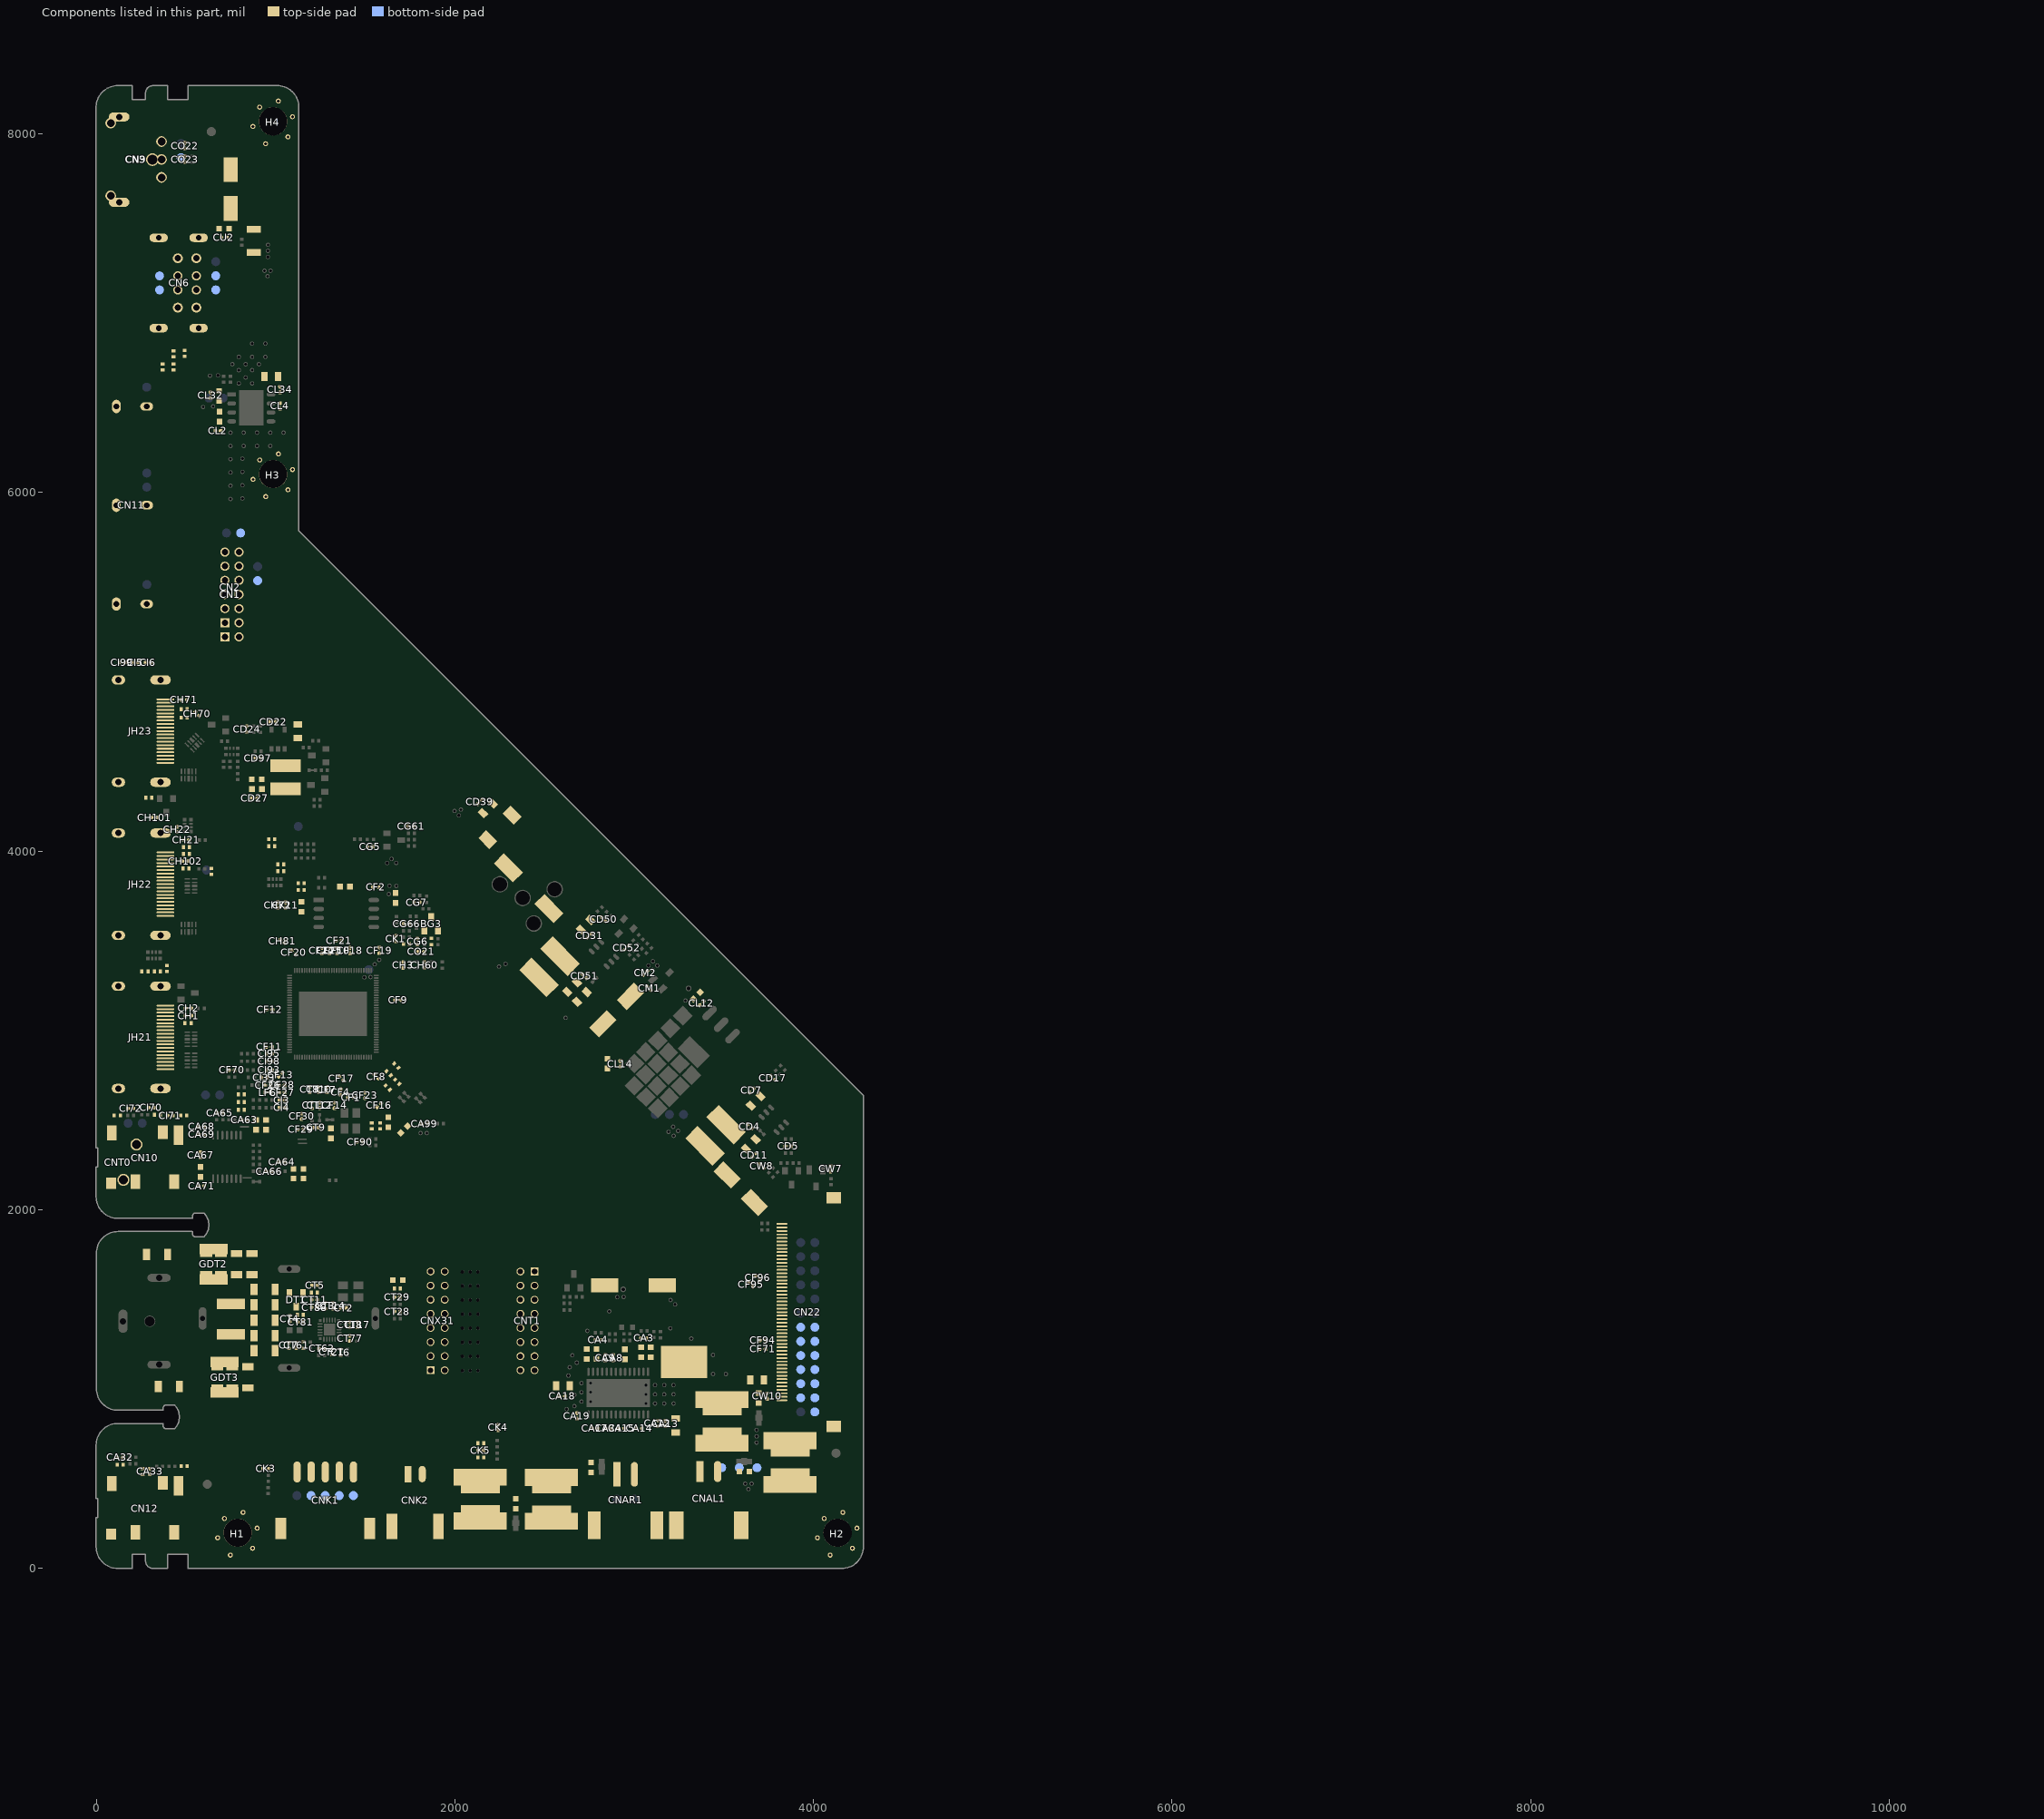
[diagram p0: the components of this part, seen from the top]
# Altium PCB MISC105950.PcbDoc (part 2 of 15)
Units mil, origin at the board's own origin, x right, y up, seen from the top; angles counter-clockwise.
Board outline 4280.62 x 8272.76 mil, 2 copper layers (TopLayer, BottomLayer), stack 61.855 mil thick; 541 components, 268 nets, 2324 pads, 1157 vias.

## Components (designator, comment, footprint, x,y, rotation, side; value= is the part's Value field where it differs from the comment) (continued)
BG3 "NC/General-purpose transistor, Dynatron, NPN, 0.2A, 40V, 30-300, SOT-23, MMBT3904(f≥350MHz), BLUE ROCKET" SOT-23 1866.5,3595 r180 top
BLON "TEST" TP 803.5,5774.51 r90 bottom
CA1 "Ceramic capacitor, CAP MC, 25V, 10uF, ±10%, X5R, 0805, SMD, TP" C0805 3231,795 r270 top
CA2 "NC/Ceramic capacitor, CAP MC, 25V, 10uF, ±10%, X5R, 0805, SMD, TP" C0805 2601.5,1017 r180 top
CA3 "3300pF-0402-X7R-±10%-50V" C0402 3053,1282.5 r0 top
CA4 "3300pF-0402-X7R-±10%-50V" C0402 2799.02,1273.23 r0 top
CA5 "Ceramic capacitor, CAP MC, 25V, 0.22uF, ±10%, X7R, 0603, SMD, TP" C0603 3092,1204 r270 top
CA6 "Ceramic capacitor, CAP MC, 25V, 0.22uF, ±10%, X7R, 0603, SMD, TP" C0603 3038,1204 r270 top
CA7 "Ceramic capacitor, CAP MC, 25V, 1uF, ±10%, X5R, 0603, SMD, TP" C0603 2947,1192.5 r90 top
CA8 "1uF-0402-X5R-±20%-16V" C0402 2881.84,1172.5 r270 top
CA9 "NC/1uF-0402-X5R-±20%-16V" C0402 2837.44,1172.5 r270 top
CA10 "Ceramic capacitor, CAP MC, 25V, 0.22uF, ±10%, X7R, 0603, SMD, TP" C0603 2788.94,1193.5 r270 top
CA11 "Ceramic capacitor, CAP MC, 25V, 0.22uF, ±10%, X7R, 0603, SMD, TP" C0603 2734.94,1193.5 r270 top
CA12 "NC/Ceramic capacitor, CAP MC, 25V, 0.1uF, ±20%, X5R, 0402, SMD, TP" C0402 3130.5,806.5 r270 top
CA13 "1000pF-0402-X7R-±10%-50V" C0402 3173,806.16 r270 top
CA14 "0.22uF-0402-X5R-±10%-16V" C0402 3027,779 r180 top
CA15 "0.22uF-0402-X5R-±10%-16V" C0402 2929,779 r0 top
CA17 "0.22uF-0402-X5R-±10%-16V" C0402 2781,779 r0 top
CA18 "NC/Ceramic capacitor, CAP MC, 25V, 0.1uF, ±20%, X5R, 0402, SMD, TP" C0402 2598.5,958.5 r180 top
CA19 "1000pF-0402-X7R-±10%-50V" C0402 2680,848.5 r270 top
CA20 "Ceramic capacitor, CAP MC, 25V, 1uF, ±10%, X5R, 0603, SMD, TP" C0603 3693.5,947.5 r270 top
CA21 "Ceramic capacitor, CAP MC, 25V, 1uF, ±10%, X5R, 0603, SMD, TP" C0603 3613.5,537.5 r180 top
CA22 "Ceramic capacitor, CAP MC, 25V, 1uF, ±10%, X5R, 0603, SMD, TP" C0603 2759,561 r270 top
CA23 "Ceramic capacitor, CAP MC, 25V, 1uF, ±10%, X5R, 0603, SMD, TP" C0603 2339.05,359 r90 top
CA29 "Ceramic capacitor, CAP MC, 6.3V, 22uF, ±20%, X5R, 0603, SMD, TP" C0603 1125.98,2226.34 r0 top
CA31 "NC/NC/Ceramic capacitor, CAP MC, 6.3V, 10uF, ±20%, X5R, 0603, SMD, TP" C0603 917.13,2445 r0 top
CA32 "NC/6800pF-0402-X7R-±10%-50V" C0402 131.5,617 r180 top
CA33 "NC/6800pF-0402-X7R-±10%-50V" C0402 297,538.5 r90 top
CA34 "0.22uF-0402-X5R-±10%-16V" C0402 2855.5,779 r180 top
CA59 "NC/NC/Ceramic capacitor, CAP MC, 6.3V, 10uF, ±20%, X5R, 0603, SMD, TP" C0603 1125.98,2172.75 r0 top
CA60 "Ceramic capacitor, CAP MC, 6.3V, 22uF, ±20%, X5R, 0603, SMD, TP" C0603 917.13,2499.75 r0 top
CA63 "NC/1uF-0402-X5R-±20%-6.3V" C0402 824.77,2501 r180 top
CA64 "NC/1uF-0402-X5R-±20%-6.3V" C0402 1035,2266 r180 top
CA65 "NC/NC/?" C0402 688,2539.5 r180 top
CA66 "NC/NC/?" C0402 962.74,2213.5 r180 top
CA67 "NC/1uF-0402-X5R-±20%-6.3V" C0402 580,2304 r90 top
CA68 "NC/1uF-0402-X5R-±20%-6.3V" C0402 585.66,2461.69 r180 top
CA69 "NC/0.1uF-0402-X7R-±10%-16V" C0402 585.66,2420 r180 top
CA70 "NC/Ceramic capacitor, CAP MC, 6.3V, 10uF, ±20%, X5R, 0603, SMD, TP" C0603 579.5,2209.88 r90 top
CA71 "NC/0.1uF-0402-X5R-±20%-16V" C0402 585.35,2131.5 r180 top
CA99 "Ceramic capacitor, CAP MC, 6.3V, 1uF, ±20%, X5R, 0402, SMD, TP" C0402 1829.35,2478.5 r180 top
CD4 "NC/0.1uF-0402-X7R-±10%-16V" C0402 3643.54,2463.96 r315 top
CD5 "NC/Ceramic capacitor, CAP MC, 50V, 1000pF, ±10%, X7R, 0402, SMD, TP" C0402 3858.27,2353.5 r180 top
CD7 "NC/NC/Ceramic capacitor, CAP MC, 25V, 0.1uF, ±20%, X5R, 0402, SMD, TP" C0402 3654.54,2664.04 r45 top
CD11 "NC/NC/0.1uF-0402-X5R-±20%-16V" C0402 3669.5,2303.5 r225 top
CD17 "NC/NC/Ceramic capacitor, CAP MC, 25V, 0.1uF, ±20%, X5R, 0402, SMD, TP" C0402 3773.5,2734.5 r315 top
CD22 "NC/0.1uF-0402-X5R-±20%-16V" C0402 984.65,4721.5 r0 top
CD24 "NC/3300pF-0402-X7R-±10%-50V" C0402 838,4680.5 r270 top
CD25 "10uF-0603-X5R-±20%-6.3V" C0603 893.69,4399.5 r0 top
CD26 "10uF-0603-X5R-±20%-6.3V" C0603 894.75,4345.41 r0 top
CD27 "NC/0.1uF-0402-X5R-±20%-16V" C0402 882.15,4295.5 r0 top
CD30 "Ceramic capacitor, CAP MC, 25V, 10uF, ±10%, X5R, 0805, SMD, TP" C0805 2728,3588.5 r225 top
CD31 "NC/Ceramic capacitor, CAP MC, 25V, 0.1uF, ±20%, X5R, 0402, SMD, TP" C0402 2749,3527.5 r45 top
CD39 "NC/Ceramic capacitor, CAP MC, 25V, 0.1uF, ±20%, X5R, 0402, SMD, TP" C0402 2138.5,4274.5 r225 top
CD50 "NC/Ceramic capacitor, CAP MC, 25V, 0.1uF, ±20%, X5R, 0402, SMD, TP" C0402 2829,3619 r315 top
CD51 "0.1uF-0402-X7R-±10%-16V" C0402 2721.5,3302 r315 top
CD52 "Ceramic capacitor, CAP MC, 50V, 1000pF, ±10%, X7R, 0402, SMD, TP" C0402 2956.72,3460.1 r45 top
CD53 "10uF-0805-X5R-±20%-16V" C0805 2653.1,3240.4 r45 top
CD54 "10uF-0805-X5R-±20%-16V" C0805 1123,4667.97 r270 top
CD57 "NC/10uF-0805-X5R-±20%-16V" C0805 2707.1,3186.4 r45 top
CD77 "NC/Ceramic capacitor, CAP MC, 25V, 10uF, ±10%, X5R, 0805, SMD, TP" C0805 3676.65,2605.35 r225 top
CD96 "NC/Ceramic capacitor, CAP MC, 25V, 10uF, ±10%, X5R, 0805, SMD, TP" C0805 2183,4238 r45 top
CD97 "Ceramic capacitor, CAP MC, 6.3V, 1uF, ±20%, X5R, 0402, SMD, TP" C0402 900.77,4517.5 r180 top
CD99 "NC/10uF-0805-X5R-±20%-16V" C0805 3650.22,2365.78 r45 top
CD101 "NC?" DIODE-S0402 1141,3821 r180 top
CD102 "NC?" DIODE-S0402 1141,3783 r180 top
CF1 "20pF-0402-NPO-±5%-50V" C0402 1417.66,2625 r180 top
CF2 "0.1uF-0402-X7R-±10%-16V" C0402 1558,3798 r180 top
CF3 "10uF-0603-X5R-±20%-6.3V" C0603 1386,3802 r180 top
CF4 "20pF-0402-NPO-±5%-50V" C0402 1361.5,2655.65 r90 top
CF5 "NC/10uF-0603-X5R-±20%-6.3V" C0603 1142.5,3689.5 r90 top
CF6 "NC/10uF-0603-X5R-±20%-6.3V" C0603 1307,2424.69 r270 top
CF7 "0.1uF-0402-X7R-±10%-16V" C0402 1285.5,2668.15 r90 top
CF8 "0.1uF-0402-X7R-±10%-16V" C0402 1561.5,2741.5 r135 top
CF9 "0.1uF-0402-X7R-±10%-16V" C0402 1681.5,3168.5 r180 top
CF10 "0.1uF-0402-X7R-±10%-16V" C0402 1341.5,3444.34 r270 top
CF11 "0.1uF-0402-X7R-±10%-16V" C0402 963.27,2907 r180 top
CF12 "0.1uF-0402-X7R-±10%-16V" C0402 965.5,3115.5 r0 top
CF13 "0.1uF-0402-X7R-±10%-16V" C0402 1026.5,2752 r45 top
CF14 "0.1uF-0402-X7R-±10%-16V" C0402 1326.5,2580.74 r90 top
CF15 "NC/10uF-0603-X5R-±20%-6.3V" C0603 1668,3738 r90 top
CF16 "0.1uF-0402-X7R-±10%-16V" C0402 1575.96,2581.46 r45 top
CF17 "0.1uF-0402-X7R-±10%-16V" C0402 1365.5,2731.5 r135 top
CF18 "0.1uF-0402-X7R-±10%-16V" C0402 1414,3444.5 r90 top
CF19 "0.1uF-0402-X7R-±10%-16V" C0402 1577,3446 r90 top
CF20 "0.1uF-0402-X7R-±10%-16V" C0402 1099.67,3434.33 r315 top
CF21 "Ceramic capacitor, CAP MC, 6.3V, 1uF, ±20%, X5R, 0402, SMD, TP" C0402 1352.16,3500.5 r180 top
CF23 "Ceramic capacitor, CAP MC, 6.3V, 1uF, ±20%, X5R, 0402, SMD, TP" C0402 1497,2637.5 r90 top
CF24 "Ceramic capacitor, CAP MC, 6.3V, 1uF, ±20%, X5R, 0402, SMD, TP" C0402 1257,3444.34 r270 top
CF25 "Ceramic capacitor, CAP MC, 6.3V, 2.2uF, ±20%, X5R, 0402, SMD, TP" C0402 1299.5,3444.34 r90 top
CF26 "0.047uF-0402-X7R-±10%-16V" C0402 956,2693.5 r180 top
CF27 "NC/0.1uF-0402-X7R-±10%-16V" C0402 1035,2652.5 r0 top
CF28 "1uF-0402-X5R-±20%-6.3V" C0402 1035,2694.5 r0 top
CF29 "NC/1000pF-0402-X7R-±10%-50V" C0402 1139.5,2447 r0 top
CF30 "NC/1000pF-0402-X7R-±10%-50V" C0402 1144.5,2520.23 r90 top
CF58 "NC/10uF-0603-X5R-±20%-6.3V" C0603 1627.5,2486.5 r90 top
CF59 "NC/10uF-0603-X5R-±20%-6.3V" C0603 1715.67,2446.67 r45 top
CF70 "0.047uF-0402-X7R-±10%-16V" C0402 755,2778 r180 top
CF71 "NC/5pF-0402-NPO-±5%-50V" C0402 3716.51,1221.48 r180 top
CF90 "NC/1000pF-0402-X7R-±10%-50V" C0402 1469,2377 r180 top
CF94 "NC/5pF-0402-NPO-±5%-50V" C0402 3716.51,1270.18 r180 top
CF95 "NC/5.6pF-0402-NPO-±5%-50V" C0402 3650.86,1582.01 r135 top
CF96 "NC/5.6pF-0402-NPO-±5%-50V" C0402 3688.62,1619.48 r135 top
CG5 "NC/0.1uF-0402-X7R-±10%-16V" C0402 1525.5,4024 r180 top
CG6 "NC/NC/0.1uF-0402-X7R-±10%-16V" C0402 1789.5,3495.5 r270 top
CG7 "NC/NC/0.1uF-0402-X7R-±10%-16V" C0402 1786,3714 r0 top
CG61 "NC/0.1uF-0402-X7R-±10%-16V" C0402 1754,4138.5 r0 top
CG66 "NC/Ceramic capacitor, CAP MC, 50V, 100pF, ±5%, NPO, 0402, SMD, TP" C0402 1729,3595 r0 top
CH1 "NC/0.1uF-0402-X7R-±10%-16V" C0402 512.5,3081 r0 top
CH2 "NC/0.1uF-0402-X7R-±10%-16V" C0402 512.5,3123 r180 top
CH3 "NC/?" C0402 1709.5,3363.5 r270 top
CH21 "NC/0.1uF-0402-X7R-±10%-16V" C0402 500.35,4062.1 r180 top
CH22 "NC/0.1uF-0402-X7R-±10%-16V" C0402 449.5,4121.5 r90 top
CH60 "NC/?" C0402 1828.5,3364.5 r270 top
CH70 "NC/0.1uF-0402-X7R-±10%-16V" C0402 561.51,4764.99 r315 top
CH71 "NC/0.1uF-0402-X7R-±10%-16V" C0402 488.5,4843.5 r0 top
CH72 "NC/?" C0402 1011.5,3698.39 r270 top
CH81 "Ceramic capacitor, CAP MC, 6.3V, 1uF, ±20%, X5R, 0402, SMD, TP" C0402 1037,3497 r315 top
CH101 "NC/10pF-0402-NPO-±5%-50V" C0402 322.65,4187.5 r0 top
CH102 "NC/10pF-0402-NPO-±5%-50V" C0402 493.84,3943.6 r180 top
CI3 "1uF-0402-X5R-±20%-6.3V" C0402 1035,2610 r180 top
CI4 "1uF-0402-X5R-±20%-6.3V" C0402 1035,2568 r180 top
CI5 "NC/10pF-0402-NPO-±5%-50V" C0402 217,5052 r180 top
CI6 "NC/10pF-0402-NPO-±5%-50V" C0402 288.5,5052 r180 top
CI33 "0.047uF-0402-X7R-±10%-16V" C0402 935.5,2736.5 r0 top
CI70 "NC/10pF-0402-NPO-±5%-50V" C0402 305,2568.5 r0 top
CI71 "NC/10pF-0402-NPO-±5%-50V" C0402 411,2524.5 r0 top
CI72 "NC/10pF-0402-NPO-±5%-50V" C0402 190.5,2564 r180 top
CI93 "0.047uF-0402-X7R-±10%-16V" C0402 963.5,2778.5 r0 top
CI95 "0.047uF-0402-X7R-±10%-16V" C0402 963.5,2869 r0 top
CI98 "0.047uF-0402-X7R-±10%-16V" C0402 963.5,2827.5 r0 top
CI99 "NC/10pF-0402-NPO-±5%-50V" C0402 143.5,5052 r180 top
CK1 "Ceramic capacitor, CAP MC, 50V, 470pF, ±5%, NPO, 0402, SMD, TP" C0402 1670,3511 r270 top
CK3 "0.1uF-0402-X7R-±10%-16V" C0402 945,554.5 r180 top
CK4 "NC/NC/0.1uF-0402-X5R-±20%-16V" C0402 2240,784.5 r270 top
CK5 "NC/0.1uF-0402-X7R-±10%-16V" C0402 2143,656.5 r180 top
CK11 "0.01uF-0402-X7R-±10%-50V" C0402 1053.5,3698.4 r270 top
CL1 "NC/Ceramic capacitor, CAP MC, 10V, 10uF, ±20%, X5R, 0603, SMD, TP" C0603 685.5,6423.5 r270 top
CL2 "0.1uF-0402-X7R-±10%-16V" C0402 678,6345 r0 top
CL4 "Ceramic capacitor, CAP MC, 16V, 1uF, ±20%, X5R, 0402, SMD, TP" C0402 1023.5,6483 r90 top
CL10 "NC/10uF-0805-X5R-±20%-16V" C0805 975,6647 r180 top
CL11 "NC/Ceramic capacitor, CAP MC, 10V, 10uF, ±20%, X5R, 0603, SMD, TP" C0603 3348,3193 r225 top
CL12 "0.1uF-0402-X7R-±10%-16V" C0402 3376,3150.5 r225 top
CL13 "NC/10uF-0603-X5R-±20%-6.3V" C0603 2849.5,2814 r270 top
CL14 "1uF-0402-X5R-±20%-6.3V" C0402 2921.5,2813 r270 top
CL31 "NC/Ceramic capacitor, CAP MC, 10V, 10uF, ±20%, X5R, 0603, SMD, TP" C0603 683.93,6539.26 r90 top
CL32 "0.1uF-0402-X7R-±10%-16V" C0402 635.43,6543.26 r90 top
CL34 "Ceramic capacitor, CAP MC, 16V, 1uF, ±20%, X5R, 0402, SMD, TP" C0402 1023.5,6574.5 r90 top
CM1 "0.1uF-0402-X7R-±10%-16V" C0402 3082.69,3234.09 r315 top
CM2 "NC/0.1uF-0402-X5R-±20%-16V" C0402 3061.5,3320 r45 top
CN1 "连接插座,connect jack,2×7PIN,D2.0,L,SNAP,STEP,Fool-proofing,Nature,L=2.5,SMD,PHD-2*7AW-DK-SMT-P,XFE" SIP2*7H/2.0D-LS 746.61,5431.32 r90 top locked
CN2 "NC/Connector socket, connect jack, 2×6PIN, D2.0, L, SNAP, STEP, Fool-proofing, Nature, L=2.5, SMD, PHD-2*6AW-DK-SMT-P, XFE-D" SIP2*6H/2.0D-LS 746.61,5470.69 r90 top locked
CN3 "NC/RCA jack, RCA Jack, AV1, H, Orange, CH5.5, Seal, SMD, RCA-143P1-EP-07, CS" AV1-H-4-S -0.01,7857.76 r270 top locked
CN6 "USB jack, USB Receptacle, USB2.0, H, Double, Black, flange, Block up, SMD, WLUS-392A, WLCO" USB2-HS-1 19.69,7169.3 r270 top locked
CN9 "Optical jack, OPTICAL, H, SMD, 182500122, VAST" OPTICAL-HS-1 0,7858.27 r270 top locked
CN10 "Earphone jack, Earphone Jack, H, Φ3.5, CH2.25, Black, switch, Seal, SMD, PJ-342F, JSL" PHONE-HS-29 0,2291.34 r270 top locked
CN11 "RCA jack, RCA Jack, AV3, H, Yellow, White, Red, CH5.5, D14, Seal, SMD, AV3-8.4-18A, JSL" AV3-H14-15-S 0,5929.14 r270 top locked
CN12 "Earphone jack, Earphone Jack, H, Φ3.5, CH2.25, Black, switch, Seal, SMD, PJ-342F, JSL" PHONE-HS-29 0,334.65 r270 top locked
CN22 "FFC connector, FFC connector, 51Pin, D0.5, Bottom, lock, SMD, CT" FFC51H/0.5S-8 3968.12,1427.35 r90 top locked
CNAL1 "Connector socket, connect jack, 2pin, D2.5, L, SNAP, Fool-proofing, Nature, L=2.4mm, SMD, AMA" SIP2H/2.5S-4 3415.5,483.06 r0 top locked
CNAR1 "Connector socket, 2PIN, D2.5, L, SNAP, Fool-proofing, RED, SMD, XFE" SIP2H/2.5S-3 2951.5,483 r0 top locked
CNK1 "Connector socket, connect jack, 5pin, D2.0, L, SNAP, STEP, Fool-proofing, Nature, L=2.5mm, SMD, AMA" SIP5H/2.0S-4 1275.9,378.02 r0 top locked
CNK2 "Connector socket, Connect jack, 2Pin, D2.0, L, SNAP, STEP, Fool-proofing, Nature, L=2.5mm, SMD, S2015-02R2WA-KSY, XYDT" SIP2H/2.0S-3 1777.21,378.02 r0 top locked
CNT0 "NC/Standoff, Φ5.5×7.0×7.8mm-M3, nickel-plated, iron, SMT" FIX-5.5*7.0*7.8-S-1 0,2263.84 r270 top locked
CNT1 "Connector socket, connect jack, 2×8Pin, D2.0, L, Fool-proofing, Black, L=2.6, DIP, JN-2.0-2*8PW-H=5.6-PC=2.6-SK, XFE" SIP2*8H/2.0DM-1 2403.84,1378.52 r270 top locked
CNX31 "Connector socket-female, female connect jack, 2×8Pin, D2.0, L, Fool-proofing, Black, L=2.6, DIP, PM-2.0-2*8PW-H=6.35-SK-AC, XFE" SIP2*8H/2.0DF-1 1902.58,1378.58 r90 top locked
CO21 "NC/33pF-0402-NPO-±5%-50V" C0402 1811,3438.5 r180 top
CO22 "NC/0.1uF-0402-X5R-±20%-16V" C0402 493,7935.38 r270 top
CO23 "NC/330pF-0402-NPO-±5%-50V" C0402 493,7858.88 r90 top
COAX "TEST" TP 470.87,7868.64 r180 bottom
CQC "CQC" CQC 1921,252.5 r0 top
CT1 "0.1uF-0402-X7R-±10%-16V" C0402 1201.5,2581.74 r270 top
CT2 "NC/Ceramic capacitor, CAP MC, 50V, 27pF, ±5%, NPO, 0402, SMD, TP" C0402 1377,1451 r180 top
CT3 "0.1uF-0402-X7R-±10%-16V" C0402 1276,1463 r270 top
CT4 "Thick-film resistor, RES, 1/16W, 0ohm, ±1%, 0402, SMD" C0402 1077.5,1390.5 r90 top
CT5 "NC/0.1uF-0402-X7R-±10%-16V" C0402 1217.5,1577 r180 top
CT6 "NC/22pF-0402-NPO-±5%-50V" C0402 1361.5,1203.5 r90 top
CT7 "Thick-film resistor, RES, 1/16W, 0ohm, ±1%, 0402, SMD" C0402 1072.5,1242.5 r90 top
CT8 "NC/47pF-0402-NPO-±5%-50V" C0402 1189,2669.5 r90 top
CT9 "NC/0.1uF-0402-X7R-±10%-16V" C0402 1223.35,2457 r180 top
CT10 "NC/47pF-0402-NPO-±5%-50V" C0402 1241,2669.5 r270 top
CT11 "Ceramic capacitor, CAP MC, 50V, 1000pF, ±10%, X7R, 0402, SMD, TP" C0402 1214.99,1496.4 r180 top
CT12 "0.1uF-0402-X7R-±10%-16V" C0402 1244,2581.74 r270 top
CT14 "NC/Ceramic capacitor, CAP MC, 50V, 27pF, ±5%, NPO, 0402, SMD, TP" C0402 1318,1463 r270 top
CT17 "NC/Ceramic capacitor, CAP MC, 50V, 1000pF, ±10%, X7R, 0402, SMD, TP" C0402 1455,1357.5 r270 top
CT18 "0.1uF-0402-X7R-±10%-16V" C0402 1412.5,1357.5 r90 top
CT21 "0.1uF-0402-X7R-±10%-16V" C0402 1313,1205.5 r270 top
CT28 "NC/47pF-0402-NPO-±5%-50V" C0402 1678,1431.5 r180 top
CT29 "NC/47pF-0402-NPO-±5%-50V" C0402 1677,1510.5 r0 top
CT40 "Ceramic capacitor, CAP MC, 1KV, 470pF, ±5%, NPO, 1206, SMD, TP" C1206 937.04,1382.38 r0 top
CT41 "Thick-film resistor, RES, 1/4W, 0ohm, ±5%, 1206, SMD" C1206 937.04,1211.52 r180 top
CT42 "Thick-film resistor, RES, 1/4W, 0ohm, ±5%, 1206, SMD" C1206 937.04,1296.96 r180 top
CT43 "Thick-film resistor, RES, 1/4W, 0ohm, ±5%, 1206, SMD" C1206 937.04,1467.84 r180 top
CT44 "Thick-film resistor, RES, 1/4W, 0ohm, ±5%, 1206, SMD" C1206 844.08,1063.91 r90 top
CT45 "NC/Ceramic capacitor, CAP MC, 1KV, 4700pF, ±10%, X7R, 1206, SMD, TP" C1206 937.04,1553.26 r0 top
CT46 "NC/Ceramic capacitor, CAP MC, 1KV, 4700pF, ±10%, X7R, 1206, SMD, TP" C1206 337.5,1748.06 r0 top
CT47 "NC/Ceramic capacitor, CAP MC, 1KV, 4700pF, ±10%, X7R, 1206, SMD, TP" C1206 781,1695.01 r90 top
CT48 "NC/Ceramic capacitor, CAP MC, 1KV, 4700pF, ±10%, X7R, 1206, SMD, TP" C1206 866,1695.01 r90 top
CT49 "NC/Ceramic capacitor, CAP MC, 1KV, 4700pF, ±10%, X7R, 1206, SMD, TP" C1206 757,1063.91 r270 top
CT50 "NC/Ceramic capacitor, CAP MC, 1KV, 4700pF, ±10%, X7R, 1206, SMD, TP" C1206 403.5,1012 r0 top (schematic designator CT46)
CT51 "NC/Ceramic capacitor, CAP MC, 1KV, 4700pF, ±10%, X7R, 1206, SMD, TP" C1206 671,1063.91 r270 top
CT52 "NC/Ceramic capacitor, CAP MC, 1KV, 4700pF, ±10%, X7R, 1206, SMD, TP" C1206 608.95,1695.01 r90 top
CT53 "NC/Ceramic capacitor, CAP MC, 1KV, 4700pF, ±10%, X7R, 1206, SMD, TP" C1206 694.5,1695.01 r90 top
CT61 "Ceramic capacitor, CAP MC, 50V, 2pF, ±0.25pF, NPO, 0402, SMD, TP" C0402 1114.5,1242.5 r90 top
CT62 "Ceramic capacitor, CAP MC, 6.3V, 1uF, ±20%, X5R, 0402, SMD, TP" C0402 1256.5,1224.5 r0 top
CT77 "NC/22pF-0402-NPO-±5%-50V" C0402 1412.5,1281.5 r90 top
CT80 "10uF-0603-X5R-±20%-6.3V" C0603 1681,1605.5 r180 top
CT81 "NC/Ceramic capacitor, CAP MC, 50V, 120pF, ±5%, NPO, 0402, SMD, TP" C0402 1137,1372.5 r0 top
CT88 "0.1uF-0402-X7R-±10%-16V" C0402 1214.99,1453.9 r0 top
CU1 "NC/10uF-0603-X5R-±20%-6.3V" C0603 711,7472.88 r0 top
CU2 "NC/Ceramic capacitor, CAP MC, 16V, 1uF, ±20%, X5R, 0402, SMD, TP" C0402 711,7423.88 r180 top
CW7 "NC/0.1uF-0402-X7R-±10%-16V" C0402 4095.5,2227 r90 top
CW8 "0.022uF-0402-X7R-±10%-16V" C0402 3710.75,2241.98 r315 top
CW9 "NC/10uF-0805-X5R-±20%-16V" C0805 3685.5,1049 r0 top
CW10 "NC/0.1uF-0402-X7R-±10%-16V" C0402 3741.5,959 r90 top
DA51 "NC/SFI0402-240E-2R5PP-LF" DIODE-S0402 488,568.5 r0 top
DA52 "NC/SFI0402-240E-2R5PP-LF" DIODE-S0402 131,576.5 r0 top
DA53 "NC/SFI0402-240E-2R5PP-LF" DIODE-S0402 256.5,539 r270 top
DAS1 "35.0*5.4mm" DOLBY_AS2 2898,1494 r90 top
DBSR "NO DOLBY" "NO DOLBY-SILK" 3421.5,2260.5 r270 bottom
DH1 "NC/SFI0402-240E-2R5PP-LF" DIODE-S0402 510.23,3040 r180 top
DH2 "NC/SFI0402-240E-2R5PP-LF" DIODE-S0402 340,3328.5 r180 top
DH3 "NC/SFI0402-240E-2R5PP-LF" DIODE-S0402 392.5,3344.5 r90 top
DH4 "NC/SFI0402-240E-2R5PP-LF" DIODE-S0402 640,3886.5 r90 top
DH21 "NC/SFI0402-240E-2R5PP-LF" DIODE-S0402 290.77,4297.5 r0 top
DH22 "NC/SFI0402-240E-2R5PP-LF" DIODE-S0402 502.06,3984.1 r180 top
DH23 "NC/SFI0402-240E-2R5PP-LF" DIODE-S0402 502.06,4022.1 r180 top
DH70 "NC/SFI0402-240E-2R5PP-LF" DIODE-S0402 498.5,3903.1 r180 top
DH71 "NC/SFI0402-240E-2R5PP-LF" DIODE-S0402 489.5,4744.5 r0 top
DH72 "NC/SFI0402-240E-2R5PP-LF" DIODE-S0402 489.5,4791.5 r0 top
DH73 "NC/TVS diode, DIO ESD, 3pF, 58V, 0402, SMD, SDV1005H260C030YPTF, Sunlord" DIODE-S0402 976.77,4065.5 r180 top
DH74 "NC/TVS diode, DIO ESD, 3pF, 58V, 0402, SMD, SDV1005H260C030YPTF, Sunlord" DIODE-S0402 976.77,4027.5 r180 top
DH75 "NC/TVS diode, DIO ESD, 3pF, 58V, 0402, SMD, SDV1005H260C030YPTF, Sunlord" DIODE-S0402 1027.27,3887.5 r180 top
DH76 "NC/TVS diode, DIO ESD, 3pF, 58V, 0402, SMD, SDV1005H260C030YPTF, Sunlord" DIODE-S0402 1027.27,3926 r180 top
DH81 "NC/SFI0402-240E-2R5PP-LF" DIODE-S0402 269.5,3328.5 r180 top
DI2 "NC/SFI0402-240E-2R5PP-LF" DIODE-S0402 807,2599 r0 top
DI3 "NC/SFI0402-240E-2R5PP-LF" DIODE-S0402 1729,3481.5 r180 top
DI22 "NC/SFI0402-240E-2R5PP-LF" DIODE-S0402 806.5,2642.5 r0 top
DI23 "NC/SFI0402-240E-2R5PP-LF" DIODE-S0402 338.5,2528.5 r180 top
DI24 "NC/SFI0402-240E-2R5PP-LF" DIODE-S0402 485.73,2524.5 r180 top
DI33 "NC/SFI0402-240E-2R5PP-LF" DIODE-S0402 806.5,2556.5 r0 top
DI34 "NC/SFI0402-240E-2R5PP-LF" DIODE-S0402 115.5,2524.5 r0 top
DIM "TEST" TP 898.43,5508.64 r180 bottom
DK2 "NC/AVLC18S02003" DIODE-S0402 1534.5,2466 r90 top
DK3 "NC/AVLC18S02003" DIODE-S0402 1581.5,2466 r90 top
DK4 "NC/ TVS diode, DIO ESD, 3pF, 58V, 0402, SMD, SDV1005H260C030YPTF, Sunlord" DIODE-S0402 2144,616.5 r180 top
DK70 "NC/TVS diode, DIO ESD, 3pF, 58V, 0402, SMD, SDV1005H260C030YPTF, Sunlord" DIODE-S0402 2144,697 r180 top
DM0 "DM0" TP 664.87,7209.38 r180 bottom
DM1 "DM0" TP 351.07,7208.88 r270 bottom
DM4 "NC/TVS diode, DIO ESD, 26.0V, SMB, SMD, SMBJ16A, GOOD-ARK" DIODE-SMB-2 2250.5,4131.5 r225 top
DO21 "NC/SFI0402-240E-2R5PP-LF" DIODE-S0402 1867.5,3495.5 r270 top
DP0 "DM0" TP 664.87,7130.64 r270 bottom
DP1 "DM0" TP 351.07,7130.14 r270 bottom
DT1 "Switching diode,DIO SW D2,200mA,100V,SOT-23,SMD,BAV99,YJ" SO-23 1113.5,1495.5 r0 top
DU1 "NC/TVS diode, DIO ESD, 0.1pF, 25V, 0402, SMD, GESD1005H150CR10GPT, Sunlord" DIODE-S0402 491,6776.38 r90 top
DU2 "NC/TVS diode, DIO ESD, 0.1pF, 25V, 0402, SMD, GESD1005H150CR10GPT, Sunlord" DIODE-S0402 429.5,6773.38 r90 top
DU11 "NC/TVS diode, DIO ESD, 0.1pF, 25V, 0402, SMD, GESD1005H150CR10GPT, Sunlord" DIODE-S0402 429.5,6701.38 r90 top
DU12 "NC/TVS diode, DIO ESD, 0.1pF, 25V, 0402, SMD, GESD1005H150CR10GPT, Sunlord" DIODE-S0402 368.5,6701.38 r90 top
DU31 "NC/TVS diode, DIO ESD, 0.1pF, 25V, 0402, SMD, GESD1005H150CR10GPT, Sunlord" DIODE-S0402 1629.56,2760.44 r315 top
DU32 "NC/TVS diode, DIO ESD, 0.1pF, 25V, 0402, SMD, GESD1005H150CR10GPT, Sunlord" DIODE-S0402 1672.5,2802.5 r315 top
DU33 "NC/TVS diode, DIO ESD, 0.1pF, 25V, 0402, SMD, GESD1005H150CR10GPT, Sunlord" DIODE-S0402 1624.5,2680 r135 top
DU34 "NC/TVS diode, DIO ESD, 0.1pF, 25V, 0402, SMD, GESD1005H150CR10GPT, Sunlord" DIODE-S0402 1677,2712.5 r135 top
E0N "TEST" TP 4007.24,1343.2 r180 bottom
E0P "TEST" TP 3928.5,1343.2 r270 bottom
E1N "TEST" TP 4007.24,1264.46 r180 bottom
E1P "TEST" TP 3928.5,1264.46 r180 bottom
E2N "TEST" TP 4007.24,1185.72 r270 bottom
E2P "TEST" TP 3928.5,1185.72 r180 bottom
E3N "TEST" TP 4007.24,1028.24 r180 bottom
E3P "TEST" TP 3928.5,1028.24 r180 bottom
E4N "TEST" TP 4007.24,949.5 r180 bottom
E4P "TEST" TP 3928.5,949.5 r180 bottom
EA1 "Aluminum electrolytic capacitor, CAP AL, 16V, 100uF, ±20%, HV, P, 6.3×5.5, SMD, TP, CapXon" EC(6.5*5.5)-S 2901.5,3112.5 r135 top
EA33 "Aluminum electrolytic capacitor, CAP AL, 25V, 470uF, ±20%, LF, RV, 10×10.5, SMD, TP, CapXon" EC(10*10.5)-S 2996.07,1577.5 r90 top locked
EA34 "Aluminum electrolytic capacitor, CAP AL, 25V, 470uF, ±20%, LF, RV, 10×10.5, SMD, TP, CapXon" EC(10*10.5)-S 2410.5,3792.5 r45 top
ECKN "TEST" TP 4007.24,1106.98 r180 bottom
ECKP "TEST" TP 3928.5,1106.98 r180 bottom
ED6 "NC/Aluminum electrolytic capacitor, CAP AL, 16V, 100uF, ±20%, HV, P, 6.3×5.5, SMD, TP, CapXon" EC(6.5*5.5)-S 3594,2116 r45 top
EU1 "Aluminum electrolytic capacitor, CAP AL, 16V, 100uF, ±20%, HV, P, 6.3×5.5, SMD, TP, CapXon" EC(6.5*5.5)-S 747,7693 r180 top
FT2 "Ferrite bead,BEAD,1000ohm,0402,300mA,SMD,TRAY,CBM100505U102T,FH" L0402 1214.21,1536.84 r0 top
FU1 "NC/NSMD110(1206-1.1A)" FUSE1.1A-S 877.38,7404 r270 top
GDT1 "NC/Gas discharge tube, GDT, 700V, 2000A, TP, 4.5×3.2mm, SMD, 4532-091-LF, Brightking" SMD4532-1 749.5,1388 r90 top
GDT2 "NC/Gas discharge tube, GDT, 700V, 2000A, TP, 4.5*3.2mm, SMD, 4532-091-LF, Brightking" SMD4532-1-C1206 653,1695 r0 top
GDT3 "NC/Gas discharge tube, GDT, 700V, 2000A, TP, 4.5*3.2mm, SMD, 4532-091-LF, Brightking" SMD4532-1-C1206 714.5,1064 r180 top
GND_AMP "DM0" TP 3487.34,559.37 r270 bottom
GND_KEY "DM0" TP 1275,403.88 r90 bottom
GND_TP "TEST" TP 4007.24,870.76 r90 bottom
H1 "Location hole" ASSE4.0C-3 787.4,196.85 r0 top locked
H2 "Location hole" ASSE4.0C-3 4133.86,196.85 r0 top locked
H3 "Location hole" ASSE4.0C-3 984.75,6102.37 r0 top locked
H4 "Location hole" ASSE4.0C-3 984.25,8070.93 r0 top locked
HS1 "Heatsink, 15.0×15.0×5.0mm, AL1060H-24, black, high-emissivity paint spray, stamped with bends, no rivet legs, YT" HS(15X15X5)-S 1318.5,3091.88 r90 top locked
HSA1 "NC/Busbar,Busbar Strip,P.CPP.200BP.2,6.0×4.0×1.0mm,T=1.0mm red copper sheet,tin-fog plated,natural color,MRD" HL030 3277.5,1149 r0 top
IR "DM0" TP 1196.26,403.88 r180 bottom
JH21 "HDMI jack, HDMI Jack, H, SMD-L, 161014162, VAST" HDMI-HS-1 -59.06,2960.63 r270 top locked
JH22 "HDMI jack, HDMI Jack, H, SMD-L, 161014162, VAST" HDMI-HS-1 -59.06,3814.96 r270 top locked
JH23 "HDMI jack, HDMI Jack, H, SMD-L, 161014162, VAST" HDMI-HS-1 -59.06,4669.29 r270 top locked
KEY "DM0" TP 1432.48,403.88 r180 bottom
LA1 "NC/Power inductor, Power Inductor, 15uH, ±20%, 2.6A, DR8.0×4.0, SMD, CKCS8040-15uH/M, CK" L(8*4.2)-S 3489.5,818 r90 top
LA2 "Power inductor, Power Inductor, 22uH, ±10%, 1.7A, 0.27×1P, DR5.8×4.5, SMD, CKO54-22uH/M-B30, CK" L(5.8*4.5)-S-3 3869,588.5 r270 top
LA3 "NC/Power inductor, Power Inductor, 15uH, ±20%, 2.6A, DR8.0×4.0, SMD, CKCS8040-15uH/M, CK" L(8*4.2)-S 3869,588.5 r270 top
LA4 "Power inductor, Power Inductor, 22uH, ±10%, 1.7A, 0.27×1P, DR5.8×4.5, SMD, CKO54-22uH/M-B30, CK" L(5.8*4.5)-S-3 2140.5,384 r90 top
LA5 "Power inductor, Power Inductor, 22uH, ±10%, 1.7A, 0.27×1P, DR5.8×4.5, SMD, CKO54-22uH/M-B30, CK" L(5.8*4.5)-S-3 3489.5,818 r90 top
LA6 "NC/Power inductor, Power Inductor, 15uH, ±20%, 2.6A, DR8.0×4.0, SMD, CKCS8040-15uH/M, CK" L(8*4.2)-S 2538,383.05 r90 top
LA7 "Power inductor, Power Inductor, 22uH, ±10%, 1.7A, 0.27×1P, DR5.8×4.5, SMD, CKO54-22uH/M-B30, CK" L(5.8*4.5)-S-3 2538,383.05 r90 top
LA8 "NC/Power inductor, Power Inductor, 15uH, ±20%, 2.6A, DR8.0×4.0, SMD, CKCS8040-15uH/M, CK" L(8*4.2)-S 2140.5,384 r90 top
LD1 "NC/Power inductor, Power Inductor, 4.7uH, ±20%, 2.8A, 0.32×1P, DR5.8×4.5, SMD, PIO54-4R7MTP02, FH" L(5.8*4.5)-S 3453.41,2414.41 r45 top
LD11 "Power inductor, Power Inductor, 4.7uH, ±20%, 2.8A, 0.32×1P, DR5.8×4.5, SMD, PIO54-4R7MTP02, FH" L(5.8*4.5)-S 2527,3354 r45 top
LD21 "Power inductor, Power Inductor, 2.2uH, ±20%, 2A, 0.28×1P, DR4.5×3.2, SMD, PIO43-2R2MTP02, FH" L(4.5*3.5)-S 1055,4411.5 r90 top
LED "DM0" TP 1353.74,403.88 r180 bottom
LF6 "NC/0ohm-0402-PCB" R0402SC#1 956.5,2653.5 r0 top
LOUT+ "DM0" TP 3684.19,559.37 r90 bottom
LOUT- "DM0" TP 3585.76,559.37 r90 bottom
LT1 "Thick-film resistor, RES, 1/16W, 0ohm, ±1%, 0402, SMD" L0402 1677.5,1559 r180 top
LT2 "NC/ Multilayer inductor, HF Inductor, 270nH, ±5%, 0402, SMD, SDCL1005CR27JTDF, Sunlord" L0402 1136.5,1413 r180 top
LT3 "Multilayer inductor, HF Inductor, 6.8nH, ±5%, 0402, SMD, MGCI1005T6N8JT-LF, Sunlord" L0402 1154.5,1243 r90 top